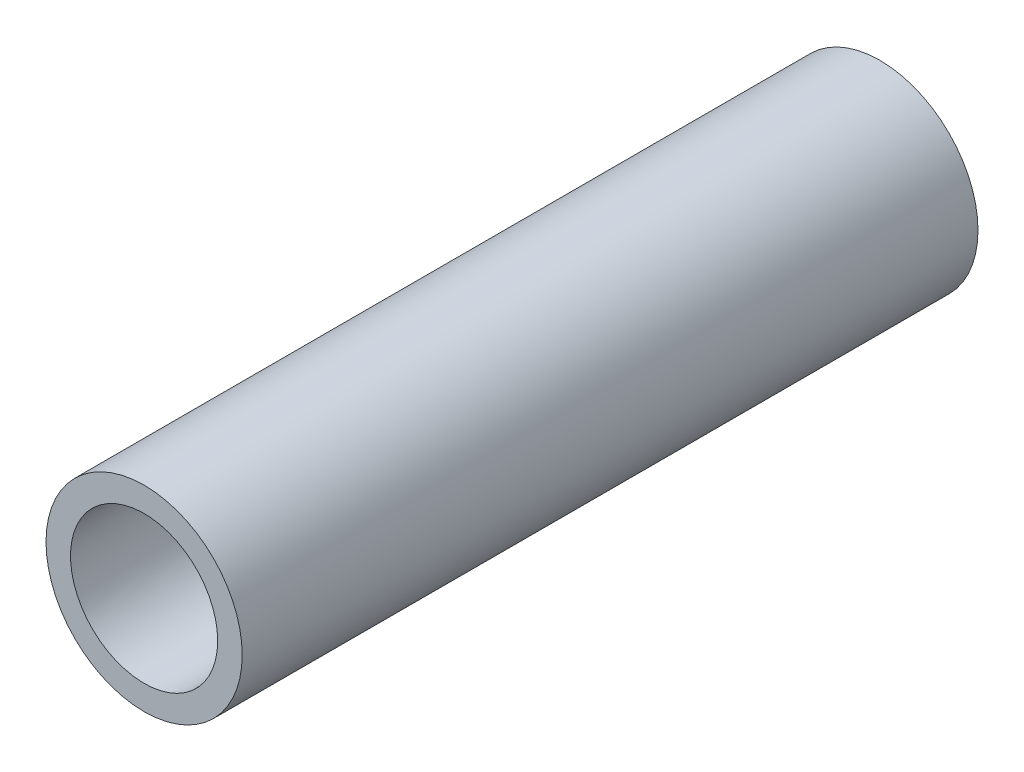
from build123d import *

# Parameters (mm, degrees)
SKETCH_1_R      = 8
SKETCH_1_R_2    = 6
EXTRUDE_1_DEPTH = 60


with BuildPart() as part:
    # 草图1 → 凸台-拉伸1 (new body)
    with BuildSketch(Plane.XY):
        Circle(SKETCH_1_R)
        Circle(SKETCH_1_R_2, mode=Mode.SUBTRACT)
    extrude(amount=EXTRUDE_1_DEPTH)


solid = part.part
